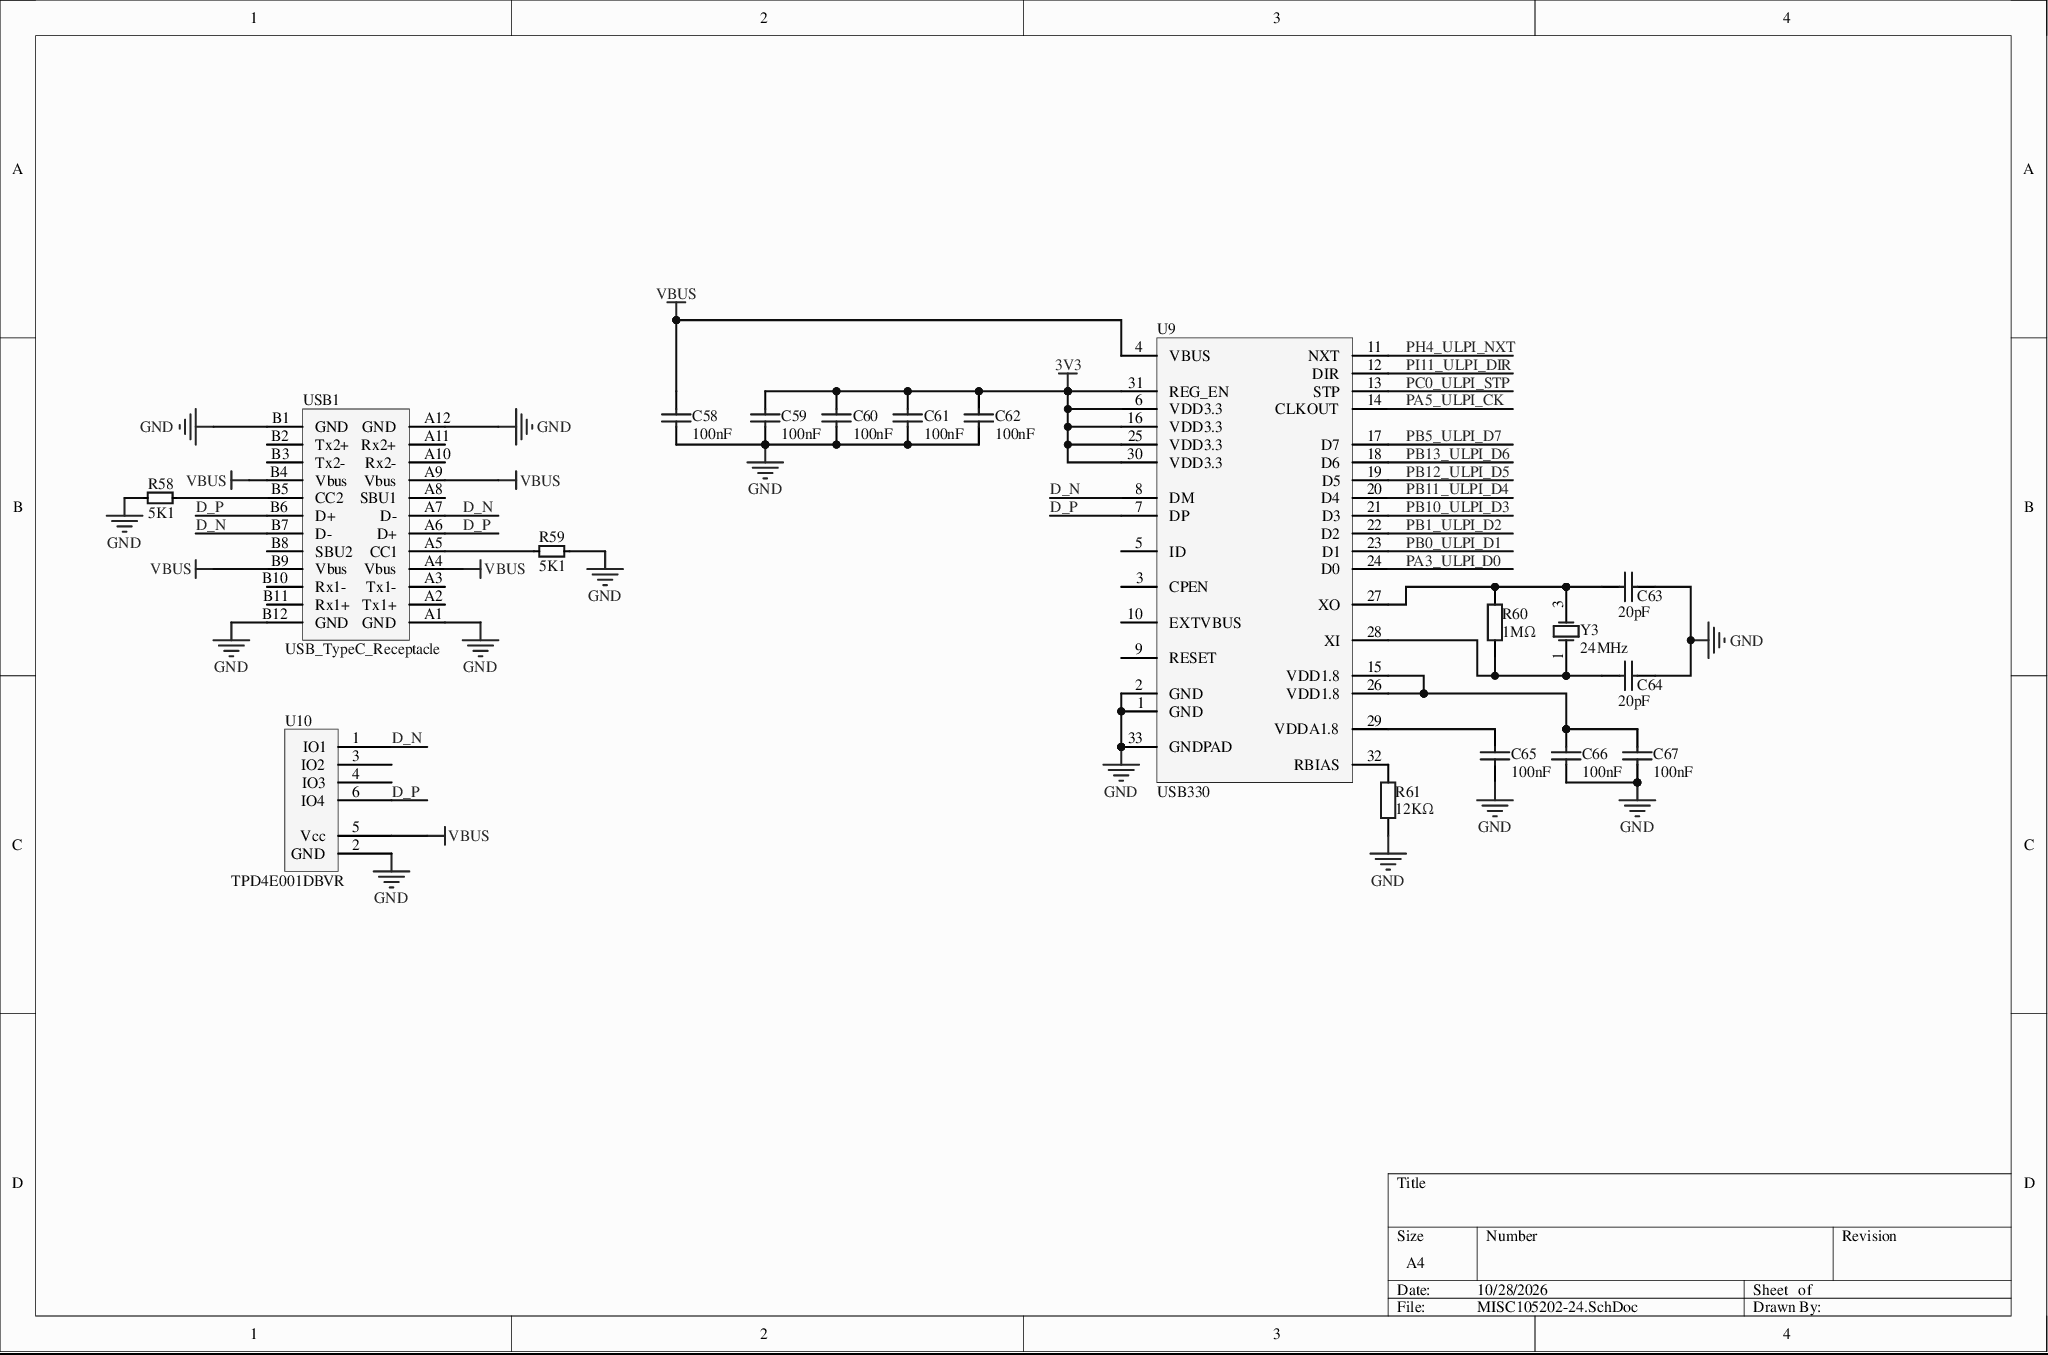
[diagram p0: MISC105202-24.SchDoc]
# Altium project MISC105202-19.PrjPCB (part 3 of 3)

## Sheet MISC105202-24.SchDoc
size A4

### Parts
C58  100nF  [0603_C]
C59  100nF  [0603_C]
C60  100nF  [0603_C]
C61  100nF  [0603_C]
C62  100nF  [0603_C]
C63  20pF  [0402_C]
C64  20pF  [0402_C]
C65  100nF  [0603_C]
C66  100nF  [0603_C]
C67  100nF  [0603_C]
R58  5K1  [0402_R]
R59  5K1  [0402_R]
R60  1MΩ  [0402_R]
R61  12KΩ  [0603_R]
U9  USB330  [QFN-32_5x5x05P]
U10  TPD4E001DBVR  [SOT-23-6]
USB1  USB_TypeC_Receptacle  [USB_TYPEC]
Y3  24MHz  [SMD-3225_4P]

### Nets
3V3: C59.2 C60.2 C61.2 C62.2 U9.6(VDD3.3) U9.16(VDD3.3) U9.25(VDD3.3) U9.30(VDD3.3) U9.31(REG_EN)
GND: C58.1 C59.1 C60.1 C61.1 C62.1 C63.2 C64.2 C65.1 C66.1 C67.1 R58.2 R59.1 R61.1 U9.1(GND) U9.2(GND) U9.33(GNDPAD) U10.2(GND) USB1.A1(GND) USB1.A12(GND) USB1.B1(GND) USB1.B12(GND)
VBUS: C58.2 U9.4(VBUS) U10.5(Vcc) USB1.A4(Vbus) USB1.A9(Vbus) USB1.B4(Vbus) USB1.B9(Vbus)
D_N: U9.8(DM) U10.1(IO1) USB1.A7(D-) USB1.B7(D-)
D_P: U9.7(DP) U10.6(IO4) USB1.A6(D+) USB1.B6(D+)
PA3_ULPI_D0: U9.24(D0)
PA5_ULPI_CK: U9.14(CLKOUT)
PB0_ULPI_D1: U9.23(D1)
PB1_ULPI_D2: U9.22(D2)
PB5_ULPI_D7: U9.17(D7)
PB10_ULPI_D3: U9.21(D3)
PB11_ULPI_D4: U9.20(D4)
PB12_ULPI_D5: U9.19(D5)
PB13_ULPI_D6: U9.18(D6)
PC0_ULPI_STP: U9.13(STP)
PH4_ULPI_NXT: U9.11(NXT)
PI11_ULPI_DIR: U9.12(DIR)
NetC63_1: C63.1 R60.2 U9.27(XO) Y3.3(OSC2)
NetC64_1: C64.1 R60.1 U9.28(XI) Y3.1(OSC1)
NetC65_2: C65.2 U9.29(VDDA1.8)
NetC66_2: C66.2 C67.2 U9.15(VDD1.8) U9.26(VDD1.8)
NetR58_1: R58.1 USB1.B5(CC2)
NetR59_2: R59.2 USB1.A5(CC1)
NetR61_2: R61.2 U9.32(RBIAS)

Not connected (* = marked no-connect by the designer): U9 3(CPEN) 5(ID) 9(RESET) 10(EXTVBUS); U10 3(IO2) 4(IO3); USB1 A2(Tx1+) A3(Tx1-) A8(SBU1) A10(Rx2-) A11(Rx2+) B2(Tx2+) B3(Tx2-) B8(SBU2) B10(Rx1-) B11(Rx1+)

### Library data of the parts
C58-C62 C65-C67 = 0603 100nF (104) 10% 50V: 贴片电容; ComponentLink1Description: supplier link; Package: 0603; Supplier: LC; SuppliersPartNumber: C14663
C63 C64 = 0402 20pF (200) 5% 50V: 贴片电容; ComponentLink1Description: supplier link; Package: 0402; Supplier: LC; SuppliersPartNumber: C1554
R58 R59 = Reszte: Resistor
R60 = 0402 1MΩ (1004) 1%: 贴片电阻; ComponentLink1Description: supplier link; Package: 0402; Supplier: LC; SuppliersPartNumber: C26083
R61 = 0603 12KΩ (1202) 1%: 贴片电阻; ComponentLink1Description: supplier link; Package: 0603; Supplier: LC; SuppliersPartNumber: C22790
U9 = USBD3300
U10 = TPD4E001
USB1 = USB_Type_C_Receptacle
Y3 = SMD-3225_4P  25MHZ 12PF 10PPM: 贴片晶振; ComponentLink1Description: supplier link; Package: SMD-3225_4P; Supplier: LC; SuppliersPartNumber: C9006

## Nets that join several sheets
3V3: MISC105202-4 (14 pins), PCBE105202 (D4.A D5.A R17.2 R19.2), MISC105202-9 (C22.2 R28.1 U5.9), MISC105202-21 (R43.1), MISC105202-13 (6 pins), MISC105202-24 (9 pins)
+5V: MISC105202-4 (P6.1), PCBE105202 (JP2.11 P8.1), MISC105202-21 (D12.1), MISC105202-13 (6 pins)
A3V3: PCBE105202 (JP2.26), MISC105202-13 (C43.2 C44.2 L1.2)
AGND: MISC105202-2 (12 pins), PCBE105202 (P3.1), MISC105202-13 (C43.1 C44.1 L2.2)
AIN2: MISC105202-2 (P1.1 R3.2), MISC105202-13 (6 pins)
GND: MISC105202-4 (15 pins), PCBE105202 (22 pins), MISC105202-9 (19 pins), MISC105202-21 (31 pins), MISC105202-13 (20 pins), MISC105202-24 (21 pins)
VBAT: PCBE105202 (JP2.16), MISC105202-13 (BT1.1)
ARM_NRST: PCBE105202 (JP3.39), MISC105202-21 (R36.2)
ARM_TCK: PCBE105202 (JP1.23 P11.2), MISC105202-21 (JP5.2)
ARM_TMS: PCBE105202 (JP1.24 P11.3), MISC105202-21 (JP6.2)
ETH_RESET: PCBE105202 (JP2.29), MISC105202-9 (R28.2 U5.15)
PA1_RMII_REF_CLK: PCBE105202 (JP3.45), MISC105202-9 (U5.14)
PA2_ETH_MDIO: PCBE105202 (JP3.43), MISC105202-9 (R29.1)
PA3_ULPI_D0: PCBE105202 (JP3.49 P3.6), MISC105202-24 (U9.24)
PA4_ADC1_CH18: MISC105202-2 (C1.2 U1.1 U1.2), PCBE105202 (JP1.25)
PA5_ULPI_CK: PCBE105202 (JP1.26 P3.3), MISC105202-24 (U9.14)
PA6_ADC2_CH3: MISC105202-2 (C5.2 U1.6 U1.7), PCBE105202 (JP1.27)
PA7_CRS_DV: PCBE105202 (JP3.42), MISC105202-9 (U5.11)
PA9_U1T: PCBE105202 (JP1.46), MISC105202-21 (P10.2 R47.1)
PA10_U1R: PCBE105202 (JP1.47), MISC105202-21 (P10.1 R46.1)
PB0_ULPI_D1: PCBE105202 (JP2.31 P3.7), MISC105202-24 (U9.23)
PB1_ULPI_D2: PCBE105202 (JP2.32 P3.8), MISC105202-24 (U9.22)
PB3_SDIO2_D2: MISC105202-4 (P6.2 R9.1), PCBE105202 (JP1.10)
PB4_SDIO2_D3: MISC105202-4 (P6.3 R8.1), PCBE105202 (JP1.9)
PB5_ULPI_D7: PCBE105202 (JP1.28 P3.13), MISC105202-24 (U9.17)
PB8_SDIO1_CKIN: MISC105202-4 (U2.1), PCBE105202 (JP1.37)
PB9_SDIO1_CDIR: MISC105202-4 (U2.4), PCBE105202 (JP1.38)
PB10_ULPI_D3: PCBE105202 (JP2.4 P3.9), MISC105202-24 (U9.21)
PB11_ULPI_D4: PCBE105202 (JP2.5 P3.10), MISC105202-24 (U9.20)
PB12_ULPI_D5: PCBE105202 (P3.11), MISC105202-24 (U9.19)
PB13_ULPI_D6: PCBE105202 (P3.12), MISC105202-24 (U9.18)
PB14_SDIO2_D0: MISC105202-4 (U2.2 U2.3), PCBE105202 (JP1.6)
PC0_ULPI_STP: PCBE105202 (P3.2), MISC105202-24 (U9.13)
PC1_ETH_MDC: PCBE105202 (JP3.44), MISC105202-9 (U5.13)
PC4_RMII_RXD0: PCBE105202 (JP3.41), MISC105202-9 (U5.8)
PC5_RMII_RXD1: PCBE105202 (JP3.40), MISC105202-9 (U5.7)
PC6_SDIO1_D0DIR: MISC105202-4 (U3.11), PCBE105202 (JP1.29)
PC7_SDIO1_ACT: MISC105202-4 (R16.1), PCBE105202 (JP1.30)
PC8_SDIO1_D0: MISC105202-4 (R12.1 TF1.7), PCBE105202 (JP1.31)
PC9_SDIO1_D1: MISC105202-4 (R13.1 TF1.8), PCBE105202 (JP1.32)
PC10_SDIO1_D2: MISC105202-4 (R11.1 TF1.1), PCBE105202 (JP1.33)
PC11_SDIO1_D3: MISC105202-4 (R14.1 TF1.2), PCBE105202 (JP1.34)
PC12_SDIO1_CK: MISC105202-4 (TF1.5), PCBE105202 (JP1.35)
PD2_SDIO1_CMD: MISC105202-4 (R15.1 TF1.3), PCBE105202 (JP1.36)
PG9_QSPI_BK2_IO2: MISC105202-4 (U3.12), PCBE105202 (JP1.16)
PG11_RMII_TX_EN: PCBE105202 (JP3.46), MISC105202-9 (U5.16)
PG12_RMII_TXD1: PCBE105202 (JP3.48), MISC105202-9 (U5.18)
PG13_RMII_TXD0: PCBE105202 (JP3.47), MISC105202-9 (U5.17)
PH4_ULPI_NXT: PCBE105202 (P3.5), MISC105202-24 (U9.11)
PI11_ULPI_DIR: PCBE105202 (JP1.44 P3.4), MISC105202-24 (U9.12)